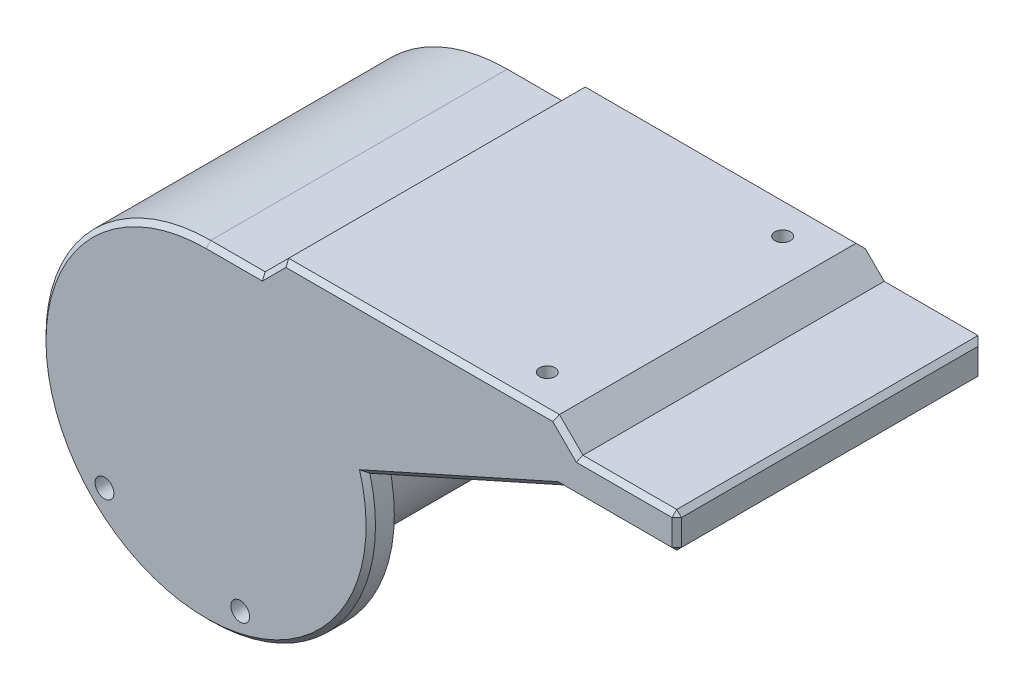
SolidWorks part; units mm, degrees
ref_plane "前视基准面" through (0, 0, 0) normal (0, 0, 1) x (1, 0, 0)
ref_plane "上视基准面" through (0, 0, 0) normal (0, 1, 0) x (1, 0, 0)
ref_plane "右视基准面" through (0, 0, 0) normal (1, 0, 0) x (0, 0, -1)
sketch "草图1" plane through (0, 0, 0) normal (0, 0, 1) x (1, 0, 0)
  circle A0 centre (0, 0) radius 52
  dimension "D1" = 104
extrude "凸台-拉伸1" add sketch "草图1" along normal mid plane 110
sketch "草图2" plane through (0, 0, 55) normal (0, 0, 1) x (1, 0, 0)
  circle A0 centre (0, 0) radius 70
  dimension "D1" = 140
extrude "凸台-拉伸2" add sketch "草图2" along normal blind 10
mirror "镜向1" about plane through (0, 0, 0) normal (0, 0, 1) of bodies 107
sketch "草图3" plane through (0, 0, -55) normal (0, 0, 1) x (1, 0, 0)
  line L0 (-67.6148, -18.1173) -> (67.6148, 18.1173)
  line L1 (0, 0) -> (-31.3921, 0) construction
  circle A0 centre (0, 0) radius 52 construction
  circle A1 centre (0, 0) radius 70
  circle A2 centre (0, 0) radius 70
  circle A3 centre (0, 0) radius 52
  circle A4 centre (0, 0) radius 70 construction
  circle M2 centre (0, 0) radius 52
  circle M3 centre (0, 0) radius 70
  dimension "D2" = 15
  dimension "D1" = 0
extrude "凸台-拉伸3" add sketch "草图3" along normal up to surface (110 mm away) contours L0 M3 M2
sketch "草图4" plane through (0, 0, 0) normal (0, 0, 1) x (1, 0, 0)
  line L0 (0, 70) -> (200, 70)
  line L1 (200, 70) -> (200, 55)
  line L2 (200, 55) -> (150, 55)
  line L3 (150, 55) -> (67.6148, 18.1173)
  line L4 (0, 70) -> (0, 0) construction
  line L5 (50.2281, 13.4586) -> (67.6148, 18.1173) construction
  line L6 (23.1228, 70) -> (33.1228, 80)
  line L7 (33.1228, 80) -> (148.152, 80)
  line L8 (148.152, 80) -> (158.152, 70)
  circle A0 centre (0, 0) radius 70 construction
  circle A1 centre (0, 0) radius 70
  dimension "D1" = 15
  dimension "D2" = 200
  dimension "D3" = 50
  dimension "D4" = 45
  dimension "D5" = 10
  dimension "D6" = 45
extrude "凸台-拉伸4" add sketch "草图4" along normal up to surface and the other way up to surface contours A1 L3 L2 L1 L0 | L8 L7 L6 L0 up to face at (70, 0, 65) other way up to face at (70, 0, -65)
sketch "草图5" plane through (0, 0, 65) normal (0, 0, 1) x (1, 0, 0)
  line L0 (0, 0) -> (-50.3538, -48.6261) construction
  line L1 (0, 0) -> (-54.9838, 0) construction
  line L2 (0, 0) -> (14.5153, -58.2177) construction
  circle A0 centre (0, 0) radius 70 construction
  circle A1 centre (-43.1604, -41.6795) radius 4
  circle A2 centre (14.5153, -58.2177) radius 4
  dimension "D2" = 60
  dimension "D3" = 8
  dimension "D5" = 60
  dimension "D1" = 44
  dimension "D4" = 60
extrude "切除-拉伸1" cut sketch "草图5" against normal blind 229
sketch "草图6" plane through (0, 80, 0) normal (0, 1, 0) x (1, 0, 0)
  circle A0 centre (130, 50) radius 3.3 construction
  circle A1 centre (130, -50) radius 3.3 construction
  circle A2 centre (130, 50) radius 3.3
  circle A3 centre (130, -50) radius 3.3
extrude "切除-拉伸2" cut sketch "草图6" against normal blind 68
sketch "草图8" plane through (0, 80, 0) normal (0, 1, 0) x (1, 0, 0)
  circle A0 centre (130, 50) radius 8
  circle A1 centre (130, -50) radius 8
  dimension "D1" = 16
extrude "切除-拉伸4" cut sketch "草图8" against normal blind 168 from offset 30 offset against normal yes
chamfer "倒角1" distance 2 angle 45 17 edges at (-42.6133, -55.5347, -65) (-42.6133, -55.5347, 65) (11.5614, 70, 65) (28.1228, 75, 65) (90.6374, 80, 65) (153.152, 75, 65) (179.076, 70, 65) (200, 70, 0) (200, 62.5, 65) (200, 55, 0) (175, 55, 65) (108.8074, 36.5587, 65) (108.8074, 36.5587, -65) (28.1228, 75, -65) (90.6374, 80, -65) (200, 62.5, -65) (175, 55, -65)
